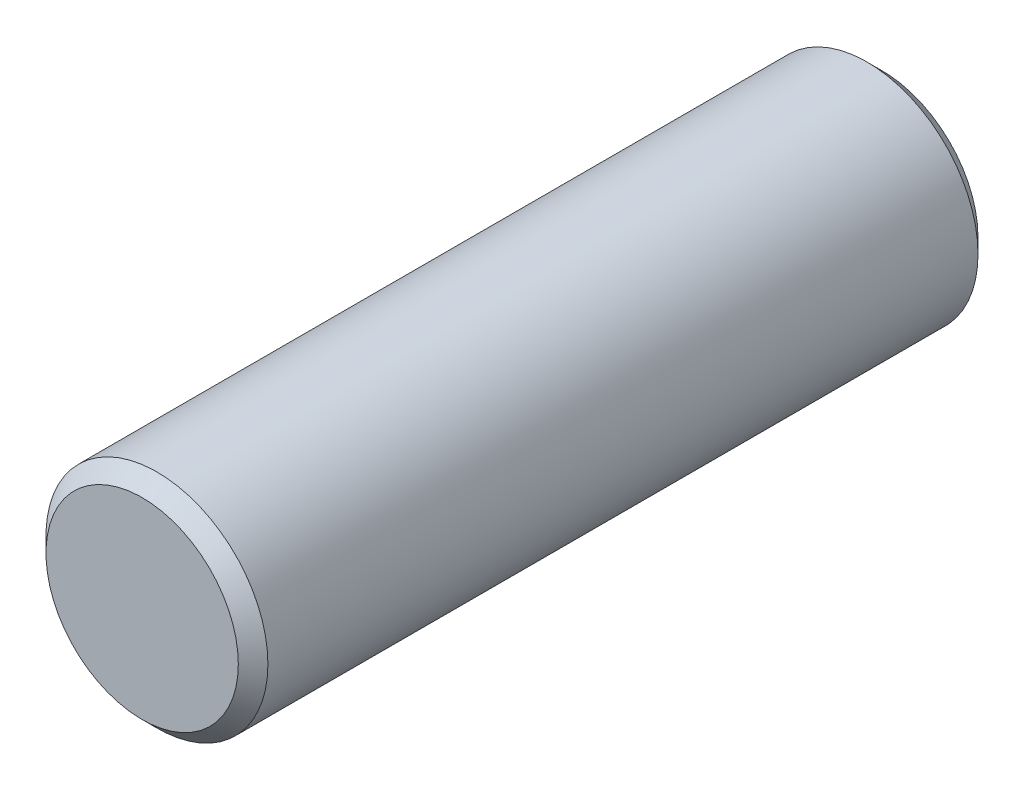
from build123d import *

# Parameters (mm, degrees)
SKETCH2_R           = 1.5
BOSS_EXTRUDE1_DEPTH = 10
CHAMFER1_SIZE       = 0.2


with BuildPart() as part:
    # Sketch2 → Boss-Extrude1 (new body)
    with BuildSketch(Plane.XY):
        with Locations((-6.262863766, 20.514795525)):
            Circle(SKETCH2_R)
    extrude(amount=-BOSS_EXTRUDE1_DEPTH)

    # Chamfer1
    chamfer1_edges = [part.edges().sort_by_distance(p)[0] for p in [
        (-7.762863766, 20.514795525, 0),
        (-7.762863766, 20.514795525, -10),
    ]]
    chamfer(chamfer1_edges, length=CHAMFER1_SIZE)


solid = part.part
